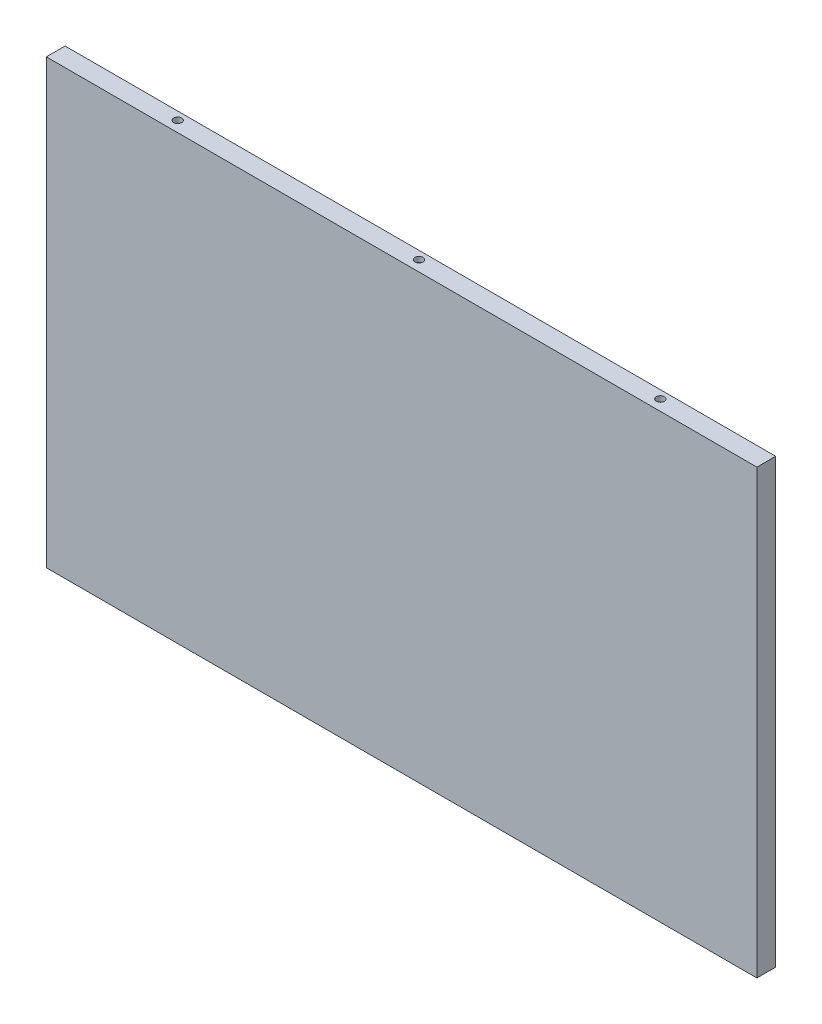
from build123d import *

# Parameters (mm, degrees)
SKETCH1_W           = 265
SKETCH1_H           = 165
BOSS_EXTRUDE1_DEPTH = 2
SKETCH2_W           = 265
SKETCH2_H           = 165
SKETCH2_W_2         = 261
SKETCH2_H_2         = 161
BOSS_EXTRUDE2_DEPTH = 5
SKETCH3_R           = 1.5
CUT_EXTRUDE1_DEPTH  = 313.209865315
LPATTERN1_COUNT     = 3
LPATTERN1_PITCH     = 90


with BuildPart() as part:
    # Sketch1 → Boss-Extrude1 (new body)
    with BuildSketch(Plane.XY):
        with Locations((132.5, 82.5)):
            Rectangle(SKETCH1_W, SKETCH1_H)
    extrude(amount=BOSS_EXTRUDE1_DEPTH)

    # Sketch2 → Boss-Extrude2 (add)
    with BuildSketch(Plane(origin=(0, 0, 0), x_dir=(-1, 0, 0), z_dir=(0, 0, -1))):
        with Locations((-132.5, 82.5)):
            Rectangle(SKETCH2_W, SKETCH2_H)
        with Locations((-132.5, 82.5)):
            Rectangle(SKETCH2_W_2, SKETCH2_H_2, mode=Mode.SUBTRACT)
    extrude(amount=BOSS_EXTRUDE2_DEPTH)

    # Sketch3 → Cut-Extrude1 (cut, through all)
    with BuildSketch(Plane(origin=(0, 165, 0), x_dir=(1, 0, 0), z_dir=(0, 1, 0))):
        with Locations(Location((225, 2, 0), (0, 0, 270))):
            Circle(SKETCH3_R)
    cut_extrude1 = extrude(amount=-CUT_EXTRUDE1_DEPTH, mode=Mode.SUBTRACT)

    # LPattern1: Cut-Extrude1 ×3
    with Locations(*[(-i * LPATTERN1_PITCH, 0, 0) for i in range(1, LPATTERN1_COUNT)]):
        add(cut_extrude1, mode=Mode.SUBTRACT)


solid = part.part
